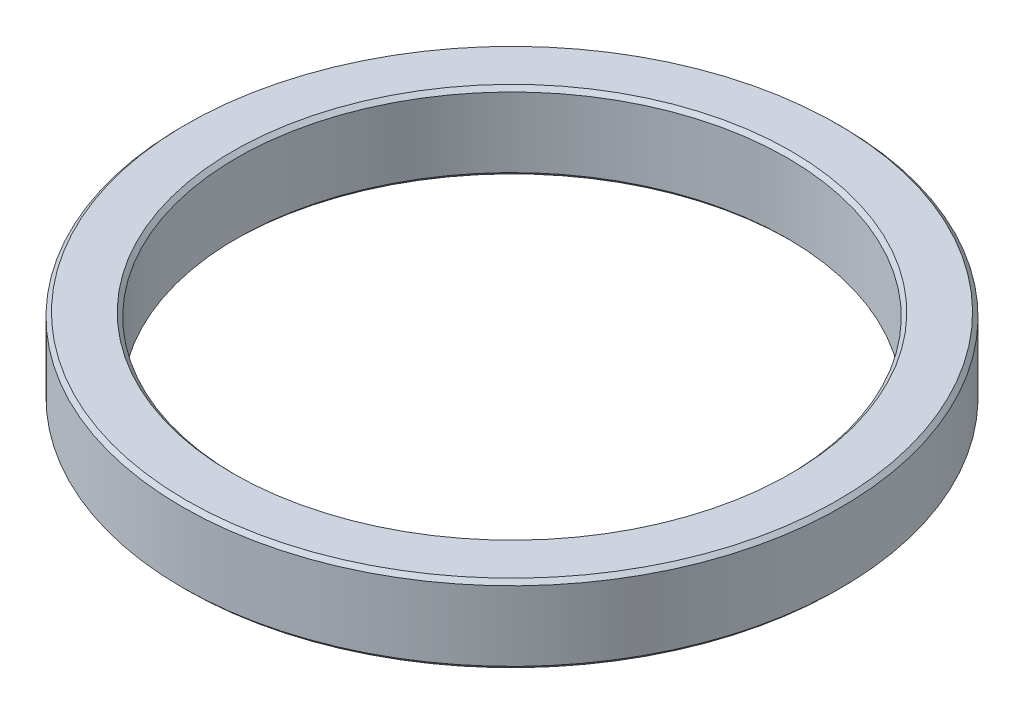
SolidWorks part; units mm, degrees
material "20 steel"
ref_plane "Front Plane" through (0, 0, 0) normal (0, 0, 1) x (1, 0, 0)
ref_plane "Top Plane" through (0, 0, 0) normal (0, 1, 0) x (1, 0, 0)
ref_plane "Right Plane" through (0, 0, 0) normal (1, 0, 0) x (0, 0, -1)
other "Configuration Table"
sketch "Sketch1" plane through (0, 0, 0) normal (0, 1, 0) x (1, 0, 0)
  circle A0 centre (0, 0) radius 42.5
  circle A1 centre (0, 0) radius 35.5
  dimension "D1" = 71
  dimension "D2" = 85
extrude "Boss-Extrude1" add sketch "Sketch1" along normal blind 10
chamfer "Chamfer2" distance 0.5 angle 45 4 edges at (0, 10, 42.5) (0, 0, 42.5) (0, 10, 35.5) (0, 0, 35.5)
